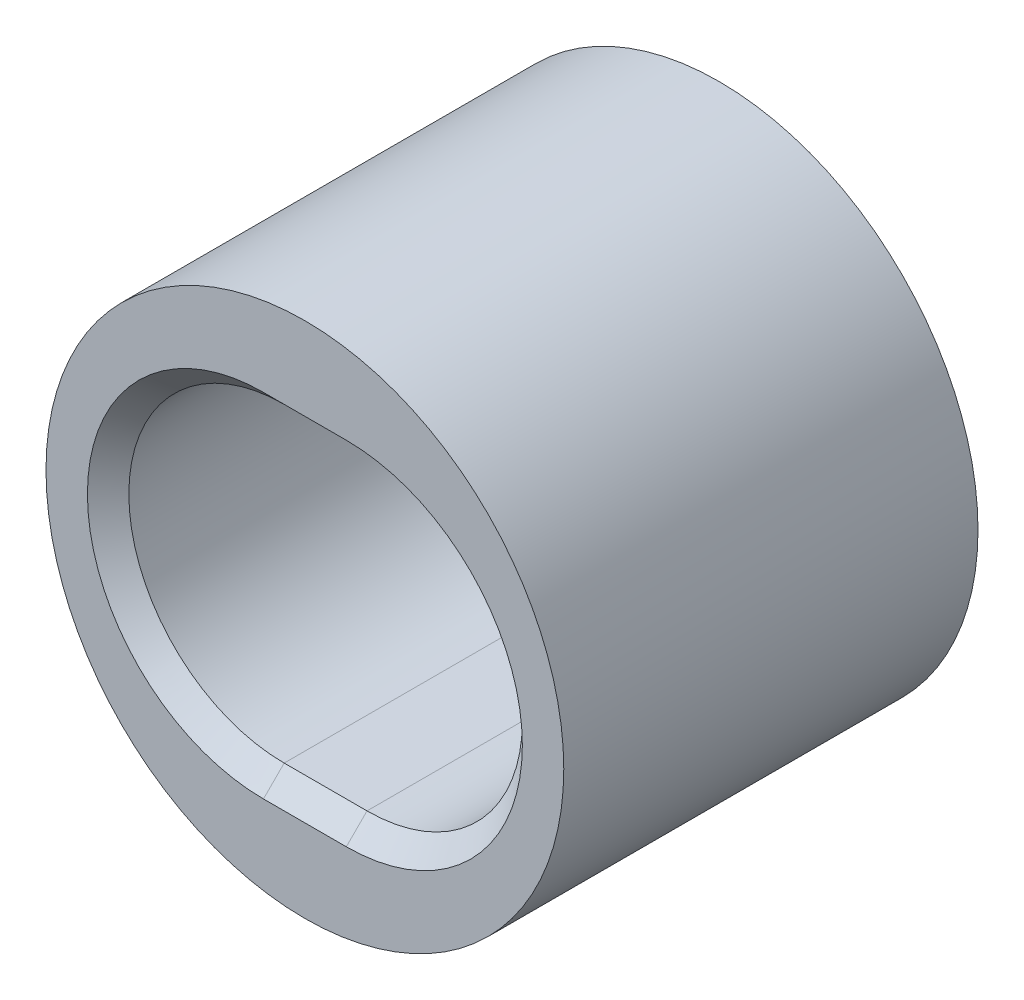
SolidWorks part; units mm, degrees
material "20#"
ref_plane "Front Plane" through (0, 0, 0) normal (0, 0, 1) x (1, 0, 0)
ref_plane "Top Plane" through (0, 0, 0) normal (0, 1, 0) x (1, 0, 0)
ref_plane "Right Plane" through (0, 0, 0) normal (1, 0, 0) x (0, 0, -1)
sketch "Sketch1" plane through (0, 0, 0) normal (0, 0, 1) x (1, 0, 0)
  line L0 (-2, 0) -> (2, 0) construction
  line L1 (-2, 7.5) -> (2, 7.5)
  line L2 (-2, -7.5) -> (2, -7.5)
  arc A0 (-2, 7.5) -> (-2, -7.5) centre (-2, 0) ccw
  circle A1 centre (0, 0) radius 12.5
  arc A2 (2, -7.5) -> (2, 7.5) centre (2, 0) ccw
  point P5 (0, 0)
  dimension "D1" = 7.5
  dimension "D3" = 25
  dimension "D2" = 4
extrude "Boss-Extrude1" add sketch "Sketch1" along normal blind 20
chamfer "Chamfer1" distance 1 angle 45 4 edges at (0, -7.5, 20) (9.5, 0, 20) (0, 7.5, 20) (-9.5, 0, 20)
